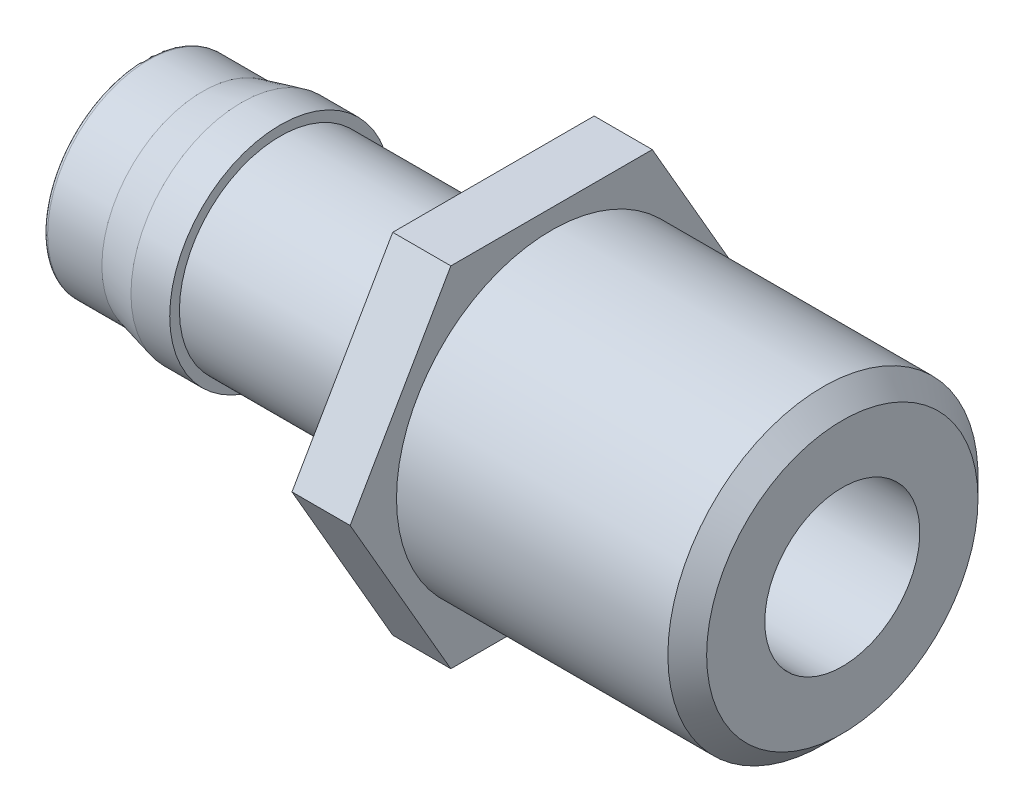
from build123d import *

# Parameters (mm, degrees)
SKETCH2_OUTSIDE_W  = 18.948
SKETCH2_OUTSIDE_H  = 18.948
CUT_EXTRUDE3_DEPTH = 10
FILLET1_R          = 0.1
CHAMFER1_SIZE      = 0.5


with BuildPart() as part:
    # Sketch1 → Revolve1 (revolve)
    with BuildSketch(Plane.XY, mode=Mode.PRIVATE) as revolve1_sk:
        Polygon((0, 2), (18, 2), (18, 4), (10.5, 4), (10.5, 6), (9, 6), (9, 2.6), (3.5, 2.6), (3.5, 2.85), (2.5, 2.85), (1.5, 2.6), (0, 2.6), align=None)
    revolve(revolve1_sk.sketch.rotate(Axis((0, 0, 0), (1, 0, 0)), 90), axis=Axis((0, 0, 0), (1, 0, 0)))

    # Sketch2 outside → Cut-Extrude3 (cut)
    with BuildSketch(Plane(origin=(10.5, 0, 0), x_dir=(0, 0, -1), z_dir=(1, 0, 0))):
        Rectangle(SKETCH2_OUTSIDE_W, SKETCH2_OUTSIDE_H)
        Polygon((2.598076211, -4.5), (5.196152423, 0), (2.598076211, 4.5), (-2.598076211, 4.5), (-5.196152423, 0), (-2.598076211, -4.5), align=None, mode=Mode.SUBTRACT)
    extrude(amount=-CUT_EXTRUDE3_DEPTH, mode=Mode.SUBTRACT)

    # Fillet1
    fillet1_edges = [part.edges().sort_by_distance(p)[0] for p in [
        (0, 0, -2.6),
    ]]
    fillet(fillet1_edges, radius=FILLET1_R)

    # Chamfer1
    chamfer1_edges = [part.edges().sort_by_distance(p)[0] for p in [
        (18, 0, -4),
    ]]
    chamfer(chamfer1_edges, length=CHAMFER1_SIZE)


solid = part.part
